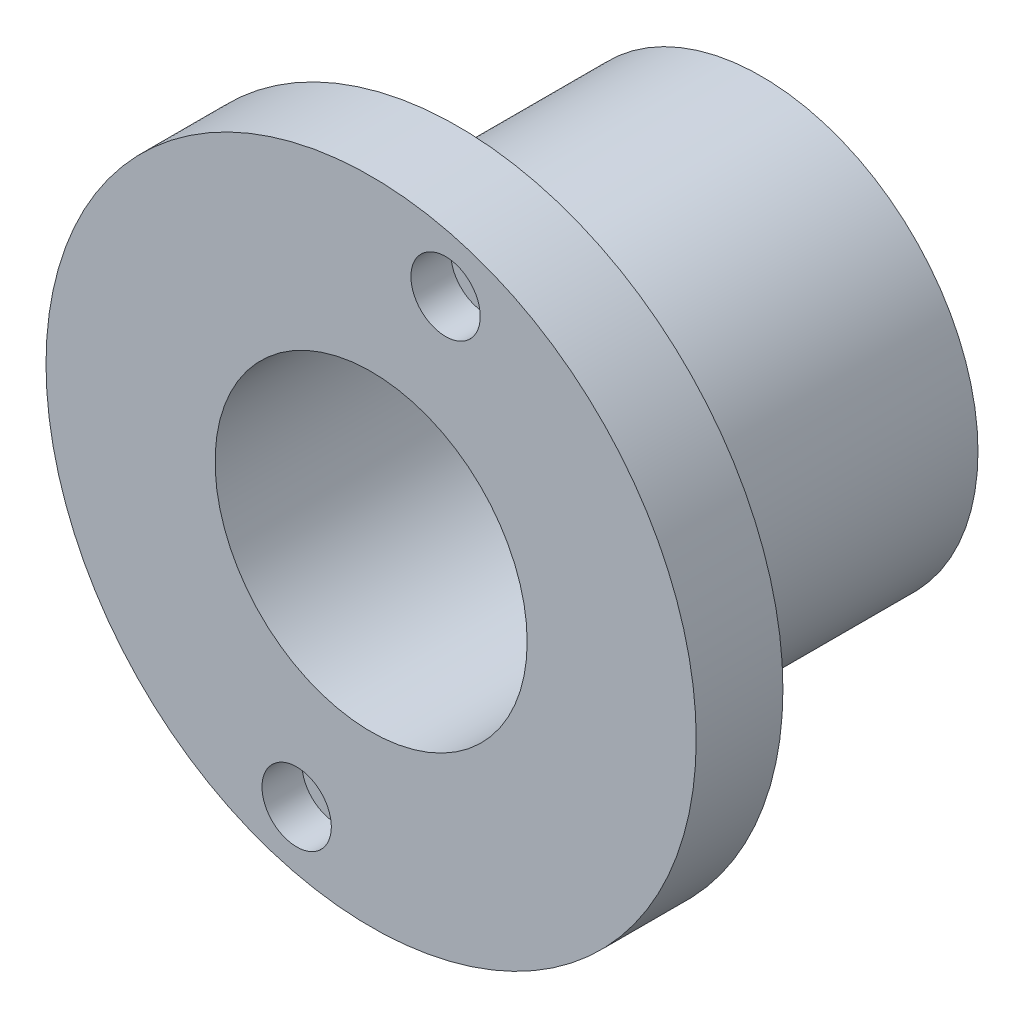
from build123d import *

# Parameters (mm, degrees)
SKETCH1_R                                            = 25
SKETCH1_R_2                                          = 18
BOSS_EXTRUDE1_DEPTH                                  = 35
SKETCH2_R                                            = 37.5
SKETCH2_R_2                                          = 18
BOSS_EXTRUDE2_DEPTH                                  = 10
HOLE_SIZE_PER_SOCKET_HEAD_CAP_SCREW_TYPE_D           = 4.5
HOLE_SIZE_PER_SOCKET_HEAD_CAP_SCREW_TYPE_CBORE_D     = 8
HOLE_SIZE_PER_SOCKET_HEAD_CAP_SCREW_TYPE_CBORE_DEPTH = 4.6


with BuildPart() as part:
    # Sketch1 → Boss-Extrude1 (new body)
    with BuildSketch(Plane.XY):
        Circle(SKETCH1_R)
        Circle(SKETCH1_R_2, mode=Mode.SUBTRACT)
    extrude(amount=BOSS_EXTRUDE1_DEPTH)

    # Sketch2 → Boss-Extrude2 (add)
    with BuildSketch(Plane.XY.offset(35)):
        Circle(SKETCH2_R)
        Circle(SKETCH2_R_2, mode=Mode.SUBTRACT)
    extrude(amount=BOSS_EXTRUDE2_DEPTH)

    # Hole size per socket head cap screw type3 (through all)
    with Locations(Plane.XY.offset(45)):
        with Locations((-8.588225841, -29.786614056), (8.588225841, 29.786614056)):
            CounterBoreHole(HOLE_SIZE_PER_SOCKET_HEAD_CAP_SCREW_TYPE_D / 2, HOLE_SIZE_PER_SOCKET_HEAD_CAP_SCREW_TYPE_CBORE_D / 2, HOLE_SIZE_PER_SOCKET_HEAD_CAP_SCREW_TYPE_CBORE_DEPTH)


solid = part.part
